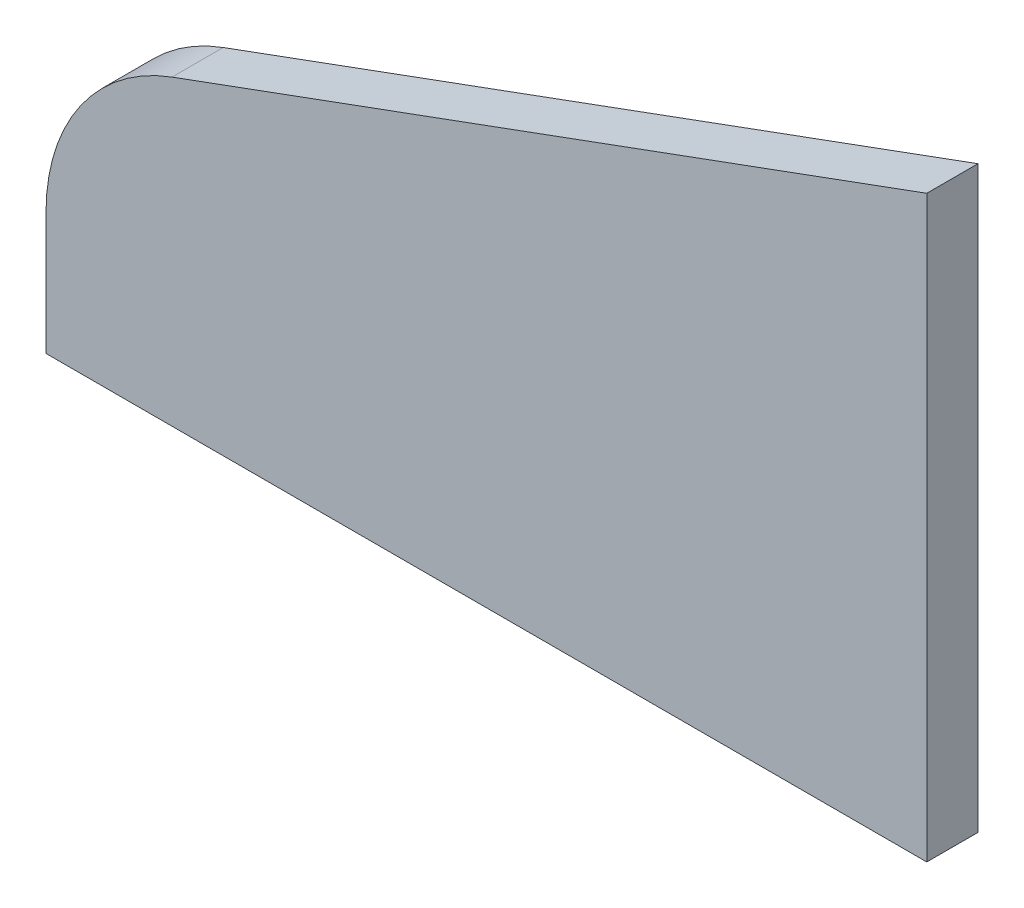
from build123d import *

# Parameters (mm, degrees)
EXTRUDE_1_DEPTH = 8


with BuildPart() as part:
    # 草图1 → 凸台-拉伸1 (new body)
    with BuildSketch(Plane(origin=(0, 0, 0), x_dir=(-1, 0, 0), z_dir=(0, 0, 1))):
        with BuildLine():
            Line((-176.477803528, -283.424824257), (-58.627916081, -240.213198859))
            ThreePointArc((-58.627916081, -240.213198859), (-44.360544026, -229.22495956), (-38.955555556, -212.046909383))
            Line((-38.955555556, -212.046909383), (-38.955555556, -193))
            Line((-38.955555556, -193), (-176.477803528, -193))
            Line((-176.477803528, -193), (-176.477803528, -283.424824257))
        make_face()
    extrude(amount=EXTRUDE_1_DEPTH)


solid = part.part
